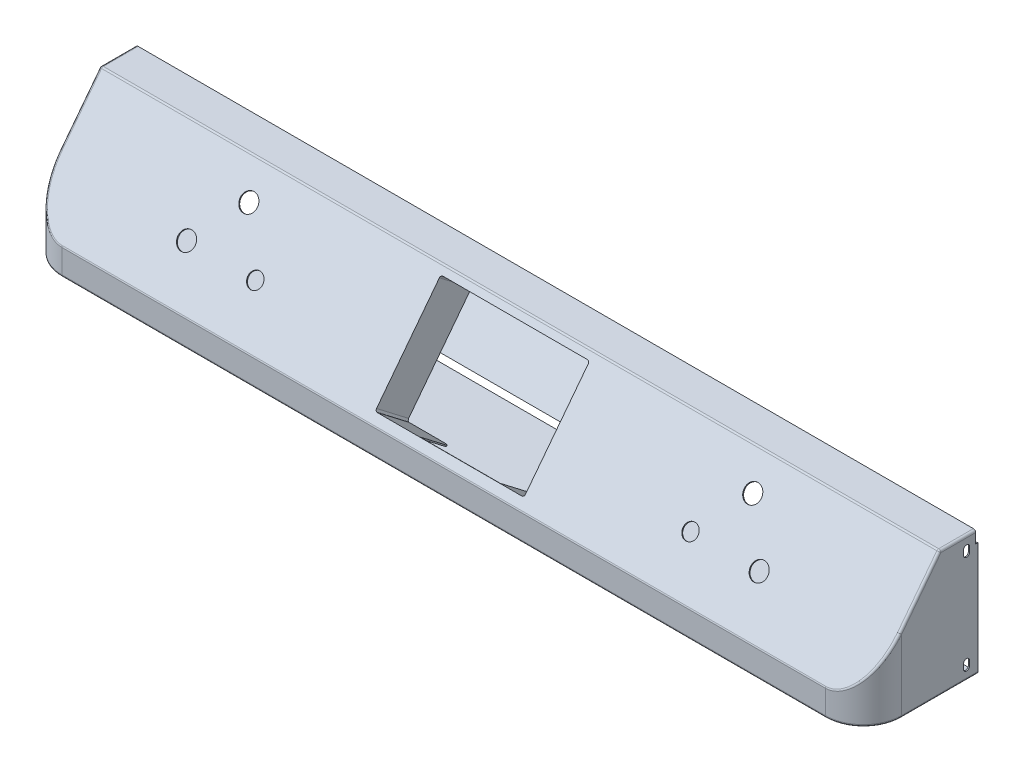
SolidWorks part; units mm, degrees
material "A3钢"
ref_plane "前视基准面" through (0, 0, 0) normal (0, 0, 1) x (1, 0, 0)
ref_plane "上视基准面" through (0, 0, 0) normal (0, 1, 0) x (1, 0, 0)
ref_plane "右视基准面" through (0, 0, 0) normal (1, 0, 0) x (0, 0, -1)
sketch "草图1" plane through (0, 0, 0) normal (0, 1, 0) x (1, 0, 0)
  line L1 (-550, 75) -> (550, 75)
  line L2 (-550, 75) -> (-550, -75)
  line L3 (-550, -75) -> (550, -75)
  line L4 (550, 75) -> (550, -75)
  line L5 (-550, 75) -> (550, -75) construction
  line L6 (-550, -75) -> (550, 75) construction
  point P0 (0, 0)
  dimension "D1" = 150
  dimension "D2" = 1100
extrude "凸台-拉伸1" add sketch "草图1" along normal blind 165
sketch "草图21" plane through (-550, 0, 0) normal (-1, 0, 0) x (0, 0, 1)
  line L0 (-25, 165) -> (75, 35)
  line L1 (-75, 165) -> (75, 165) construction
  line L2 (75, 165) -> (75, 0) construction
  line L4 (75, 35) -> (149.0161, 35)
  line L5 (149.0161, 35) -> (149.0161, 165)
  line L6 (149.0161, 165) -> (-25, 165)
  line L8 (-75, 165) -> (-75, 0) construction
  line L9 (-75, 0) -> (75, 0) construction
  dimension "D1" = 50
  dimension "D3" = 130
  dimension "D4" = 52.431
  dimension "D5" = 35
extrude "切除-拉伸8" cut sketch "草图21" against normal through all
fillet "圆角2" radius 50 2 edges at (550, 17.5, 75) (-550, 17.5, 75)
shell "抽壳1" thickness 1.5
hole_wizard "Ø8.0 (8) 直径孔1" positions "草图5" profile "草图6" hole size "Ø8.0" standard "GB" end condition through all
sketch "草图5" plane through (-550, 0, 0) normal (-1, 0, 0) x (0, 0, 1)
  line L0 (-75, 165) -> (-25, 165) construction
  line L1 (-75, 165) -> (-75, 0) construction
  line L2 (25, 0) -> (-75, 0) construction
  point P0 (-60, 147)
  point P3 (-60, 18)
  dimension "D1" = 18
  dimension "D2" = 15
  dimension "D3" = 18
sketch "草图6" plane through (-550, 147, -60) normal (0, 1, 0) x (0, 0, 1)
  line L0 (0, 0) -> (0, 1100)
  line L1 (0, 1100) -> (4, 1100)
  line L2 (4, 1100) -> (4, 0)
  line L5 (4, 0) -> (0, 0)
  line L11 (0, -6.35) -> (0, 107.95) construction
  dimension "通孔孔直径" = 8
  dimension "通孔孔深度" = 1100
sketch "草图20" plane through (-550, 0, 0) normal (-1, 0, 0) x (0, 0, 1)
  line L0 (-75, 165) -> (-75, 0) construction
  line L1 (-155.035, 190.9856) -> (-72, 190.9856)
  line L2 (-155.035, 190.9856) -> (-155.035, 149)
  line L3 (-155.035, 149) -> (-72, 149)
  line L4 (-72, 190.9856) -> (-72, 149)
  line L5 (-75, 165) -> (-25, 165) construction
  dimension "D1" = 3
  dimension "D2" = 16
extrude "切除-拉伸7" cut sketch "草图20" against normal through all
fillet "圆角5" radius 3 13 edges at (535.3553, 54.0381, 60.3553) (0, 35, 75) (-535.3553, 54.0381, 60.3553) (0, 165, -25) (-550, 132.5, 0) (550, 132.5, 0) (-550, 165, -48.5) (550, 165, -48.5) (550, 0, -25) (535.3553, 0, 60.3553) (0, 0, 75) (-535.3553, 0, 60.3553) (-550, 0, -25)
sketch "草图23" plane through (550, 0, 0) normal (1, 0, 0) x (0, 0, -1)
  line L0 (60, 150) -> (60, 144) construction
  line L1 (64, 150) -> (64, 144)
  line L2 (56, 150) -> (56, 144)
  line L3 (60, 15) -> (60, 21) construction
  line L4 (56, 15) -> (56, 21)
  line L5 (64, 15) -> (64, 21)
  arc A0 (64, 150) -> (56, 150) centre (60, 150) ccw
  arc A1 (56, 144) -> (64, 144) centre (60, 144) ccw
  arc A2 (56, 15) -> (64, 15) centre (60, 15) ccw
  arc A3 (64, 21) -> (56, 21) centre (60, 21) ccw
  circle A4 centre (60, 147) radius 4 construction
  point P2 (60, 147)
  point P9 (60, 18)
  dimension "D1" = 6
extrude "切除-拉伸10" cut sketch "草图23" against normal through all
sketch "草图24" plane through (0, 49.2565, 64.0335) normal (0, 0.6097, 0.7926) x (1, 0, 0)
  line L0 (0, 0) -> (0, 95.8156) construction
  line L1 (-94.5, 136) -> (94.5, 136)
  line L2 (-97.5, 133) -> (-97.5, -2)
  line L3 (-94.5, -5) -> (94.5, -5)
  line L4 (97.5, 133) -> (97.5, -2)
  line L5 (-97.5, 136) -> (97.5, -5) construction
  line L6 (-97.5, -5) -> (97.5, 136) construction
  arc A0 (97.5, 133) -> (94.5, 136) centre (94.5, 133) ccw
  arc A1 (97.5, -2) -> (94.5, -5) centre (94.5, -2) cw
  arc A2 (-94.5, -5) -> (-97.5, -2) centre (-94.5, -2) cw
  arc A3 (-94.5, 136) -> (-97.5, 133) centre (-94.5, 133) ccw
  point P0 (0, 65.5)
  dimension "D4" = 3
  dimension "D1" = 195
  dimension "D2" = 141
  dimension "D3" = 5
extrude "切除-拉伸11" cut sketch "草图24" against normal blind 10
sketch "草图25" plane through (0, 48.3419, 62.8445) normal (0, -0.6097, -0.7926) x (-1, 0, 0)
  line L0 (99, -2) -> (99, 133)
  line L1 (94.5, 137.5) -> (-94.5, 137.5)
  line L2 (-99, 133) -> (-99, -2)
  line L3 (-94.5, -6.5) -> (94.5, -6.5)
  line L4 (94.5, 136) -> (-94.5, 136)
  line L5 (97.5, -2) -> (97.5, 133)
  line L6 (-94.5, -5) -> (94.5, -5)
  line L7 (-97.5, 133) -> (-97.5, -2)
  line L8 (94.5, 136) -> (-94.5, 136)
  line L9 (97.5, -2) -> (97.5, 133)
  line L10 (-94.5, -5) -> (94.5, -5)
  line L11 (-97.5, 133) -> (-97.5, -2)
  arc A0 (99, 133) -> (94.5, 137.5) centre (94.5, 133) ccw
  arc A1 (-94.5, 137.5) -> (-99, 133) centre (-94.5, 133) ccw
  arc A2 (-99, -2) -> (-94.5, -6.5) centre (-94.5, -2) ccw
  arc A3 (94.5, -6.5) -> (99, -2) centre (94.5, -2) ccw
  arc A4 (-94.5, 136) -> (-97.5, 133) centre (-94.5, 133) ccw
  arc A5 (97.5, 133) -> (94.5, 136) centre (94.5, 133) ccw
  arc A6 (94.5, -5) -> (97.5, -2) centre (94.5, -2) ccw
  arc A7 (-97.5, -2) -> (-94.5, -5) centre (-94.5, -2) ccw
  arc A8 (-94.5, 136) -> (-97.5, 133) centre (-94.5, 133) ccw
  arc A9 (97.5, 133) -> (94.5, 136) centre (94.5, 133) ccw
  arc A10 (94.5, -5) -> (97.5, -2) centre (94.5, -2) ccw
  arc A11 (-97.5, -2) -> (-94.5, -5) centre (-94.5, -2) ccw
  dimension "D1" = 0
  dimension "D2" = 1.5
extrude "凸台-拉伸2" add sketch "草图25" along normal blind 51.5
sketch "草图26" plane through (0, 16.9418, 22.0244) normal (0, -0.6097, -0.7926) x (-1, 0, 0)
  line L0 (-99, 66) -> (99, 66)
  line L1 (94.5, 136) -> (-94.5, 136) construction
  line L4 (99, -2) -> (99, 133)
  line L5 (94.5, 137.5) -> (-94.5, 137.5)
  line L6 (-99, 133) -> (-99, -2)
  line L7 (-94.5, -6.5) -> (94.5, -6.5)
  line L8 (99, 66) -> (99, 133)
  line L9 (94.5, 137.5) -> (-94.5, 137.5)
  line L10 (-99, 133) -> (-99, 66)
  arc A4 (94.5, -6.5) -> (99, -2) centre (94.5, -2) ccw
  arc A5 (99, 133) -> (94.5, 137.5) centre (94.5, 133) ccw
  arc A6 (-94.5, 137.5) -> (-99, 133) centre (-94.5, 133) ccw
  arc A7 (-99, -2) -> (-94.5, -6.5) centre (-94.5, -2) ccw
  arc A9 (99, 133) -> (94.5, 137.5) centre (94.5, 133) ccw
  arc A10 (-94.5, 137.5) -> (-99, 133) centre (-94.5, 133) ccw
  dimension "D2" = 70
  dimension "D1" = 0
extrude "凸台-拉伸3" add sketch "草图26" along normal blind 1.5
sketch "草图27" plane through (0, -3.9631, 3.0486) normal (0, 0.7926, -0.6097) x (1, 0, 0)
  line L0 (0, 0) -> (0, -139.7345) construction
  line L1 (-94.5, -80.7867) -> (94.5, -80.7867) construction
  line L2 (-65, -24.3003) -> (65, -24.3003)
  line L3 (-65, -24.3003) -> (-65, -79.2867)
  line L4 (-65, -79.2867) -> (65, -79.2867)
  line L5 (65, -24.3003) -> (65, -79.2867)
  line L6 (-65, -24.3003) -> (65, -79.2867) construction
  line L7 (-65, -79.2867) -> (65, -24.3003) construction
  point P2 (0, -51.7935)
  dimension "D1" = 130
  dimension "D2" = 1.5
extrude "切除-拉伸12" cut sketch "草图27" against normal blind 1.5
other "移动面1" face at (-65, 28.0843, 45.9403) parameters "D1"=25
fillet "圆角6" radius 10 2 edges at (65, 12.3842, 25.5302) (-40, 12.3842, 25.5302)
sketch "草图28" plane through (0, 49.2565, 64.0335) normal (0, 0.6097, 0.7926) x (1, 0, 0)
  line L0 (0, 0) -> (0, 424.8692) construction
  line L1 (330, 105) -> (330, -116.4367) construction
  line L2 (-330, 105) -> (-330, -75.6643) construction
  circle A0 centre (-330, 105) radius 11.25
  circle A1 centre (330, 105) radius 11.25
  circle A2 centre (-285, 45) radius 11.25 construction
  circle A3 centre (285, 45) radius 11.25 construction
  circle A4 centre (375, 45) radius 11.25
  circle A5 centre (285, 45) radius 9.75
  circle A6 centre (-285, 45) radius 9.75
  circle A7 centre (-375, 45) radius 11.25
  dimension "D1" = 22.5
  dimension "D4" = 22.5
  dimension "D5" = 19.5
  dimension "D2" = 660
  dimension "D3" = 105
  dimension "D6" = 90
  dimension "D7" = 60
extrude "切除-拉伸13" cut sketch "草图28" against normal blind 1.5
